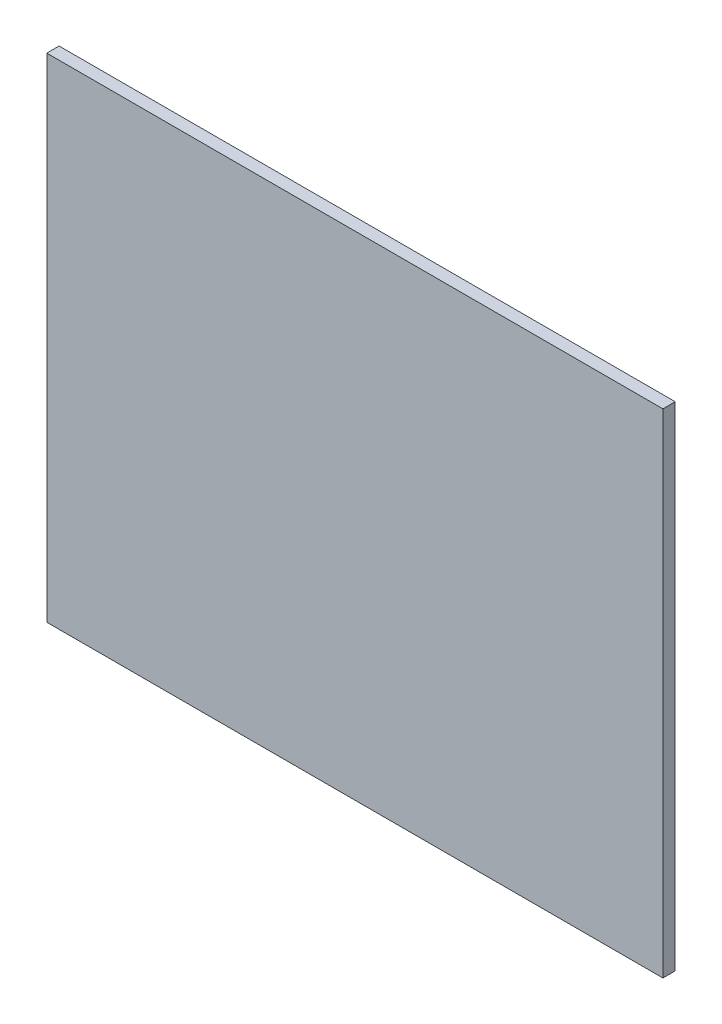
from build123d import *

# Parameters (mm, degrees)
SKETCH1_W           = 100
SKETCH1_H           = 80
BOSS_EXTRUDE1_DEPTH = 2


with BuildPart() as part:
    # Sketch1 → Boss-Extrude1 (new body)
    with BuildSketch(Plane.XY):
        Rectangle(SKETCH1_W, SKETCH1_H)
    extrude(amount=BOSS_EXTRUDE1_DEPTH)


solid = part.part
